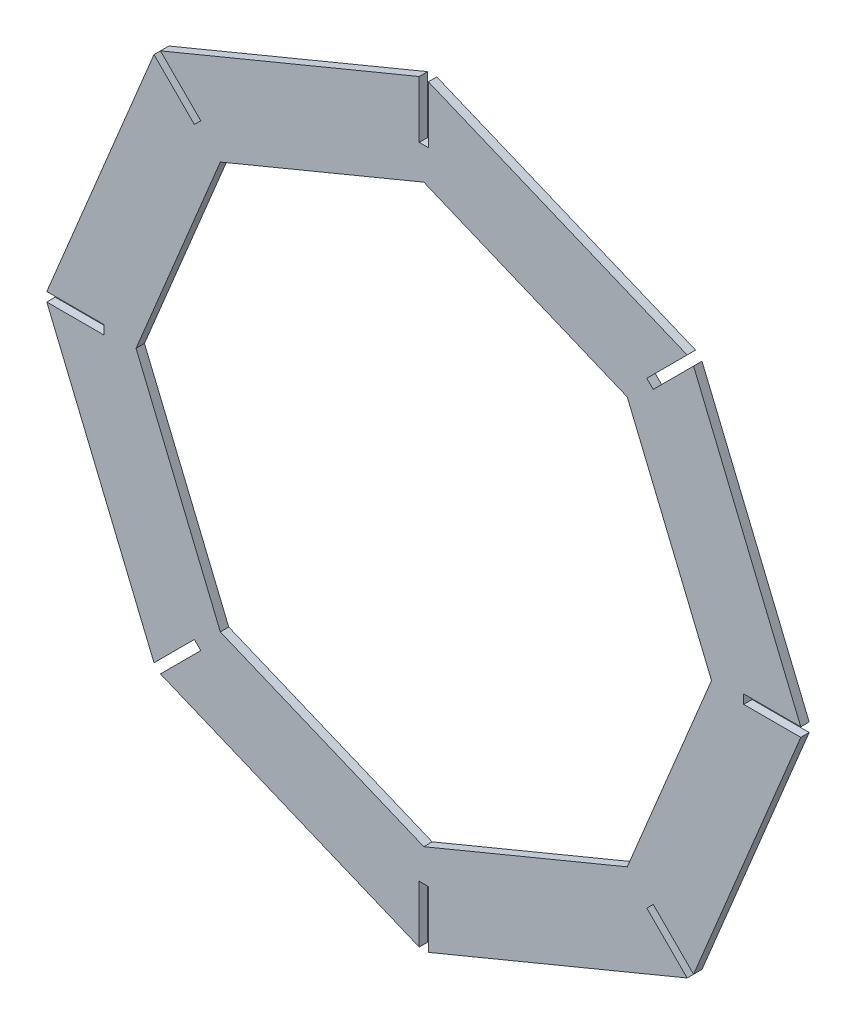
from build123d import *

# Parameters (mm, degrees)
EXTRUDE_1_DEPTH     = 5
CUT_EXTRUDE_1_DEPTH = 606
SKETCH_4_W          = 70
SKETCH_4_H          = 5.4
SKETCH_4_W_2        = 5.4
SKETCH_4_H_2        = 70
CUT_EXTRUDE_2_DEPTH = 10


with BuildPart() as part:
    # 草图1 → 凸台-拉伸1 (new body)
    with BuildSketch(Plane.XY):
        Polygon((159.099025767, 159.099025767), (0, 225), (-159.099025767, 159.099025767), (-225, 0), (-159.099025767, -159.099025767), (0, -225), (159.099025767, -159.099025767), (225, 0), align=None)
    extrude(amount=EXTRUDE_1_DEPTH)

    # 草图2 → 切除-拉伸1 (cut)
    with BuildSketch(Plane.XY.offset(5)):
        Polygon((0, 170.880389985), (-120.83068253, 120.83068253), (-170.880389985, 0), (-120.83068253, -120.83068253), (0, -170.880389985), (120.83068253, -120.83068253), (170.880389985, 0), (120.83068253, 120.83068253), align=None)
    extrude(amount=-CUT_EXTRUDE_1_DEPTH, mode=Mode.SUBTRACT)

    # 草图4 → 切除-拉伸2 (cut)
    with BuildSketch(Plane.XY.offset(5)):
        Polygon((185.756951418, -181.938574799), (136.259476735, -132.441100116), (132.441100116, -136.259476735), (181.938574799, -185.756951418), align=None)
        with Locations((225, 0)):
            Rectangle(SKETCH_4_W, SKETCH_4_H)
        with Locations((0, -225)):
            Rectangle(SKETCH_4_W_2, SKETCH_4_H_2)
        Polygon((-181.938574799, -185.756951418), (-132.441100116, -136.259476735), (-136.259476735, -132.441100116), (-185.756951418, -181.938574799), align=None)
        with Locations((-225, 0)):
            Rectangle(SKETCH_4_W, SKETCH_4_H)
        Polygon((-185.756951418, 181.938574799), (-136.259476735, 132.441100116), (-132.441100116, 136.259476735), (-181.938574799, 185.756951418), align=None)
        with Locations((0, 225)):
            Rectangle(SKETCH_4_W_2, SKETCH_4_H_2)
        Polygon((181.938574799, 185.756951418), (132.441100116, 136.259476735), (136.259476735, 132.441100116), (185.756951418, 181.938574799), align=None)
    extrude(amount=-CUT_EXTRUDE_2_DEPTH, mode=Mode.SUBTRACT)


solid = part.part
